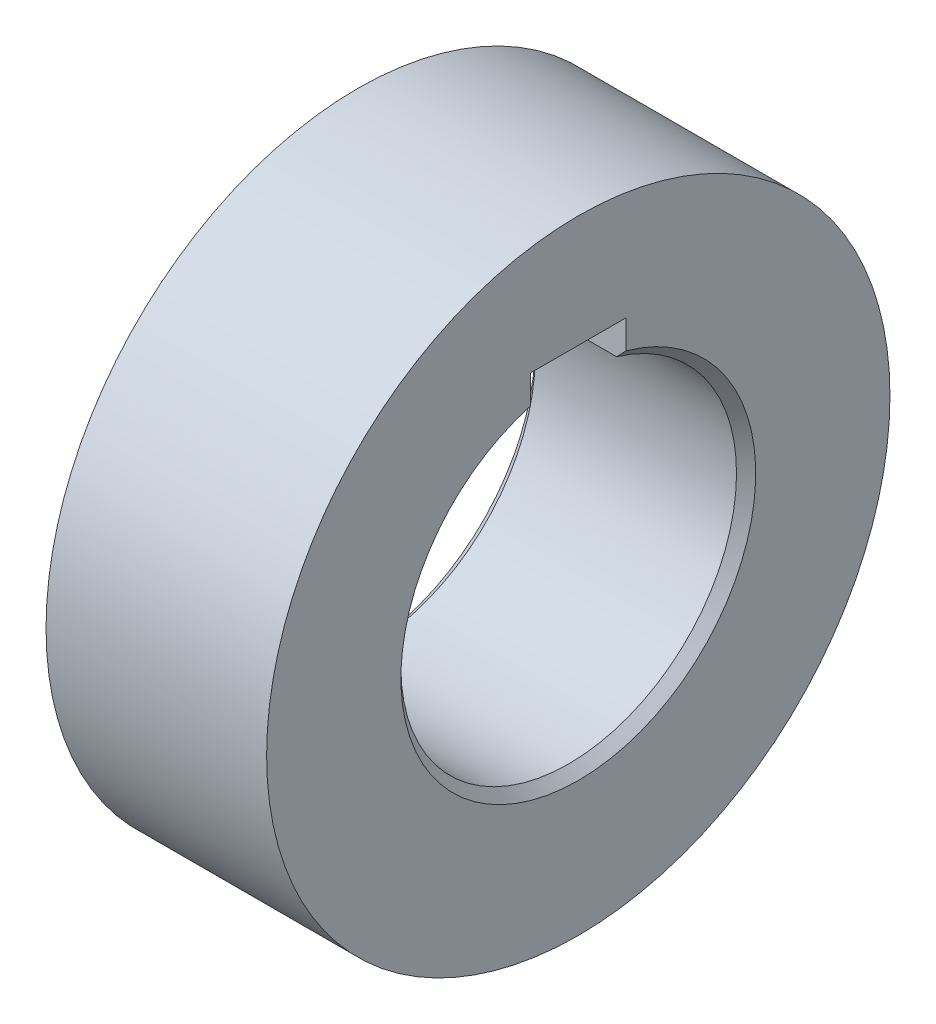
SolidWorks part; units mm, degrees
ref_plane "前视基准面" through (0, 0, 0) normal (0, 0, 1) x (1, 0, 0)
ref_plane "上视基准面" through (0, 0, 0) normal (0, 1, 0) x (1, 0, 0)
ref_plane "右视基准面" through (0, 0, 0) normal (1, 0, 0) x (0, 0, -1)
sketch "草图1" plane through (0, 0, 0) normal (0, 0, 1) x (1, 0, 0)
  line L0 (0, 0) -> (64.8368, 0) construction
  line L1 (0, 17.5) -> (0, 45.25)
  line L2 (0, 45.25) -> (18, 45.25)
  line L3 (18, 45.25) -> (18, 31.5)
  line L4 (18, 31.5) -> (23, 31.5)
  line L5 (23, 31.5) -> (23, 17.5)
  line L6 (23, 17.5) -> (0, 17.5)
  line L7 (2.6592, 45.25) -> (6.1599, 33.8) construction
  line L8 (6.1599, 33.8) -> (11.8401, 33.8) construction
  line L9 (11.8401, 33.8) -> (15.3408, 45.25) construction
  line L10 (0, 42.5) -> (18, 42.5) construction
  line L11 (9, 33.8) -> (9, 17.5) construction
  point P17 (3.5, 42.5)
  point P18 (14.5, 42.5)
  dimension "d2" = 90.5
  dimension "L" = 23
  dimension "B" = 18
  dimension "d" = 35
  dimension "d1" = 63
  dimension "dd" = 85
  dimension "f" = 9
  dimension "槽轮角" = 34
  dimension "bd" = 11
  dimension "hf" = 8.7
  dimension "ha" = 2.75
revolve "旋转1" add sketch "草图1" angle 360 about L0
sketch "草图2" plane through (0, 0, 0) normal (0, 0, 1) x (1, 0, 0)
  line L0 (11.8401, 33.8) -> (15.3408, 45.25) construction
  line L1 (6.1599, 33.8) -> (11.8401, 33.8) construction
  line L2 (2.6592, 45.25) -> (6.1599, 33.8) construction
  line L3 (11.8401, 33.8) -> (15.3408, 45.25)
  line L4 (6.1599, 33.8) -> (11.8401, 33.8)
  line L5 (2.6592, 45.25) -> (6.1599, 33.8)
  line L6 (2.6592, 45.25) -> (15.3408, 45.25)
  line L7 (0, 0) -> (18, 0) construction
  line L8 (18, -31.5) -> (18, 31.5) construction
revolve "切除-旋转1" cut sketch "草图2" angle 360 about L7
chamfer "倒角1" distance 1 2 edges at (23, 0, 17.5) (0, 0, 17.5)
sketch "草图4" plane through (0, 0, 0) normal (-1, 0, 0) x (0, 0, 1)
  line L1 (-5, 16.7705) -> (5, 16.7705)
  line L2 (-5, 16.7705) -> (-5, 20.8)
  line L3 (-5, 20.8) -> (5, 20.8)
  line L4 (5, 16.7705) -> (5, 20.8)
  circle A0 centre (0, 0) radius 17.5 construction
  point P6 (1.7, 20.8)
  dimension "键槽高度" = 20.8
  dimension "键槽宽度" = 10
  dimension "t1" = 3.3
extrude "切除-拉伸1" cut sketch "草图4" against normal through all
sketch "草图6" plane through (0, 0, 0) normal (1, 0, 0) x (0, 0, -1)
  circle A0 centre (0, 0) radius 31.5
extrude "切除-拉伸3" cut sketch "草图6" against normal blind 2 and the other way blind 23 flip side to cut
sketch "草图8" plane through (0, 0, 0) normal (1, 0, 0) x (0, 0, -1)
  circle A0 centre (0, 0) radius 31.5
sketch "草图9" plane through (0, 0, 0) normal (1, 0, 0) x (0, 0, -1)
  circle A0 centre (0, 0) radius 31.5
  circle A1 centre (0, 0) radius 32.5
extrude "凸台-拉伸1" add sketch "草图9" along normal blind 23
